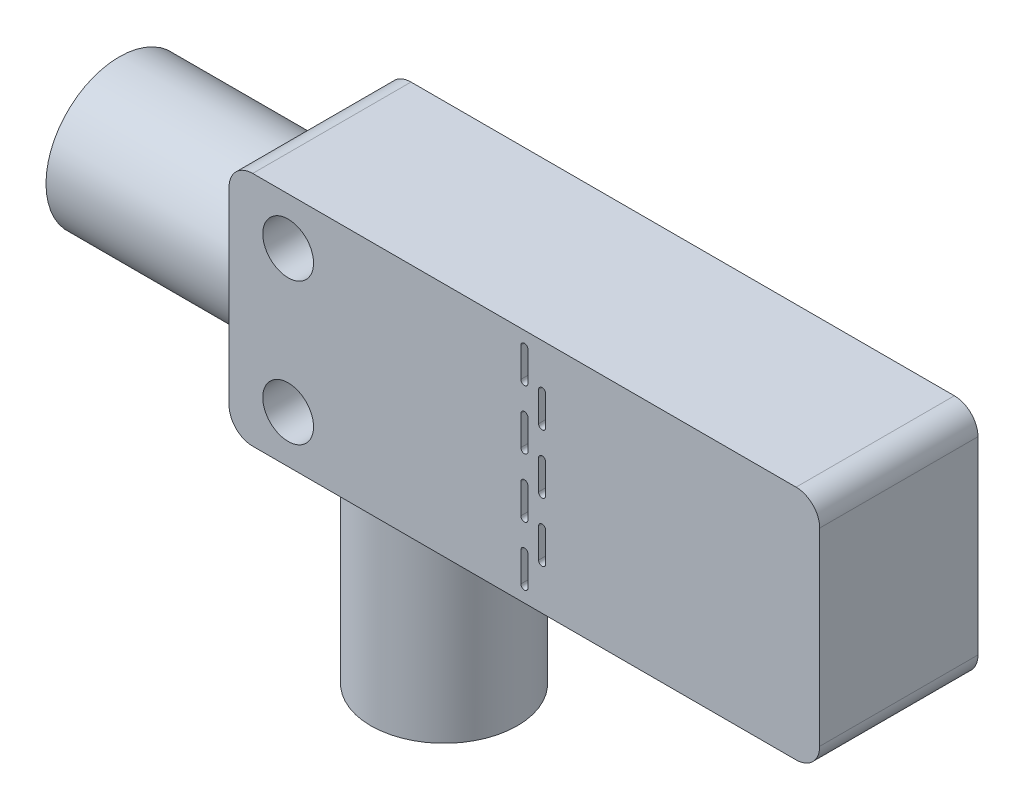
SolidWorks part; units mm, degrees
material "黑色POM"
ref_plane "前视基准面" through (0, 0, 0) normal (0, 0, 1) x (1, 0, 0)
ref_plane "上视基准面" through (0, 0, 0) normal (0, 1, 0) x (1, 0, 0)
ref_plane "右视基准面" through (0, 0, 0) normal (1, 0, 0) x (0, 0, -1)
sketch "草图1" plane through (0, 0, 0) normal (0, 0, 1) x (1, 0, 0)
  line L1 (-25, 10) -> (25, 10)
  line L2 (-25, 10) -> (-25, -10)
  line L3 (-25, -10) -> (25, -10)
  line L4 (25, 10) -> (25, -10)
  line L5 (-25, 10) -> (25, -10) construction
  line L6 (-25, -10) -> (25, 10) construction
  point P0 (0, 0)
  dimension "D1" = 20
  dimension "D2" = 50
extrude "凸台-拉伸1" add sketch "草图1" along normal blind 13.4
sketch "草图2" plane through (0, -10, 0) normal (0, -1, 0) x (1, 0, 0)
  line L0 (-25, 13.4) -> (25, 13.4) construction
  line L1 (-25, 13.4) -> (-25, 0) construction
  circle A0 centre (-13.5, 6.7) radius 6.2
  dimension "D1" = 6.7
  dimension "D2" = 11.5
extrude "凸台-拉伸2" add sketch "草图2" along normal blind 16
sketch "草图3" plane through (-25, 0, 0) normal (-1, 0, 0) x (0, 0, 1)
  line L0 (13.4, 10) -> (13.4, -10) construction
  line L1 (13.4, 10) -> (0, 10) construction
  circle A0 centre (6.7, 0) radius 6.2
  dimension "D1" = 6.7
  dimension "D2" = 10
extrude "凸台-拉伸3" add sketch "草图3" along normal blind 16
hole_wizard "Ø6.0 (6) 直径孔1" positions "草图6" profile "草图5" hole size "Ø6.0" standard "ISO"
sketch "草图6" plane through (-41, 0, 0) normal (-1, 0, 0) x (0, 0, 1)
  point P1 (6.7, 0)
sketch "草图5" plane through (-41, 0, 6.7) normal (0, 1, 0) x (0, 0, 1)
  line L0 (0, 0) -> (0, 31.8026)
  line L1 (0, 31.8026) -> (3, 30)
  line L2 (3, 30) -> (3, 0)
  line L5 (3, 0) -> (0, 0)
  line L10 (0, 31.8026) -> (-3, 30) construction
  line L11 (0, -6.35) -> (0, 107.95) construction
  dimension "孔直径" = 6
  dimension "孔深度" = 30
  dimension "导头角度" = 118
hole_wizard "Ø6.0 (6) 直径孔2" positions "草图8" profile "草图7" hole size "Ø6.0" standard "ISO"
sketch "草图8" plane through (0, -26, 0) normal (0, -1, 0) x (1, 0, 0)
  point P1 (-13.5, 6.7)
sketch "草图7" plane through (-13.5, -26, 6.7) normal (1, 0, 0) x (0, 0, -1)
  line L0 (0, 0) -> (0, 31.8026)
  line L1 (0, 31.8026) -> (3, 30)
  line L2 (3, 30) -> (3, 0)
  line L5 (3, 0) -> (0, 0)
  line L10 (0, 31.8026) -> (-3, 30) construction
  line L11 (0, -6.35) -> (0, 107.95) construction
  dimension "孔直径" = 6
  dimension "孔深度" = 30
  dimension "导头角度" = 118
hole_wizard "Ø4.3 (4.3) 直径孔1" positions "草图10" profile "草图9" hole size "Ø4.3" standard "ISO"
sketch "草图10" plane through (0, 0, 13.4) normal (0, 0, 1) x (1, 0, 0)
  line L1 (0, 0) -> (-25, 0) construction
  line L2 (-25, 10) -> (-25, -10) construction
  point P0 (-20, 6)
  point P1 (-20, -6)
  dimension "D1" = 12
  dimension "D2" = 5
sketch "草图9" plane through (-20, 6, 13.4) normal (1, 0, 0) x (0, -1, 0)
  line L0 (0, 0) -> (0, 31.2919)
  line L1 (0, 31.2919) -> (2.15, 30)
  line L2 (2.15, 30) -> (2.15, 0)
  line L5 (2.15, 0) -> (0, 0)
  line L10 (0, 31.2919) -> (-2.15, 30) construction
  line L11 (0, -6.35) -> (0, 107.95) construction
  dimension "孔直径" = 4.3
  dimension "孔深度" = 30
  dimension "导头角度" = 118
fillet "圆角1" radius 2 4 edges at (-25, -10, 6.7) (-25, 10, 6.7) (25, 10, 6.7) (25, -10, 6.7)
sketch "草图11" plane through (0, 0, 13.4) normal (0, 0, 1) x (1, 0, 0)
  line L0 (0, 8.75) -> (0, 6.25) construction
  line L1 (0.3, 8.75) -> (0.3, 6.25)
  line L2 (-0.3, 8.75) -> (-0.3, 6.25)
  line L3 (-25, 8) -> (-25, -8) construction
  line L4 (23, 10) -> (-23, 10) construction
  arc A0 (0.3, 8.75) -> (-0.3, 8.75) centre (0, 8.75) ccw
  arc A1 (-0.3, 6.25) -> (0.3, 6.25) centre (0, 6.25) ccw
  point P2 (0, 7.5)
  dimension "D1" = 25
  dimension "D2" = 1.25
  dimension "D3" = 2.5
  dimension "D4" = 0.6
extrude "切除-拉伸1" cut sketch "草图11" against normal up to next
pattern_linear "阵列(线性)1" count 4 spacing 5 along (0, -1, 0) of "切除-拉伸1"
sketch "草图12" plane through (0, 0, 13.4) normal (0, 0, 1) x (1, 0, 0)
  line L0 (0, 5.95) -> (0, 4.05) construction
  line L1 (0, 5) -> (3, 5) construction
  line L2 (1.5, 6.25) -> (1.5, 3.75) construction
  line L3 (1.8, 6.25) -> (1.8, 3.75)
  line L4 (1.2, 6.25) -> (1.2, 3.75)
  line L5 (0.3, 6.25) -> (0.3, 8.75) construction
  arc A0 (-0.3, 6.25) -> (0.3, 6.25) centre (0, 6.25) ccw construction
  arc A1 (0.3, 3.75) -> (-0.3, 3.75) centre (0, 3.75) ccw construction
  arc A2 (1.8, 6.25) -> (1.2, 6.25) centre (1.5, 6.25) ccw
  arc A3 (1.2, 3.75) -> (1.8, 3.75) centre (1.5, 3.75) ccw
  arc A4 (0.3, 8.75) -> (-0.3, 8.75) centre (0, 8.75) ccw construction
  point P12 (1.5, 5)
  dimension "D1" = 1.5
extrude "切除-拉伸2" cut sketch "草图12" against normal up to next
pattern_linear "阵列(线性)2" count 3 spacing 5 along (0, -1, 0) of "切除-拉伸2"
